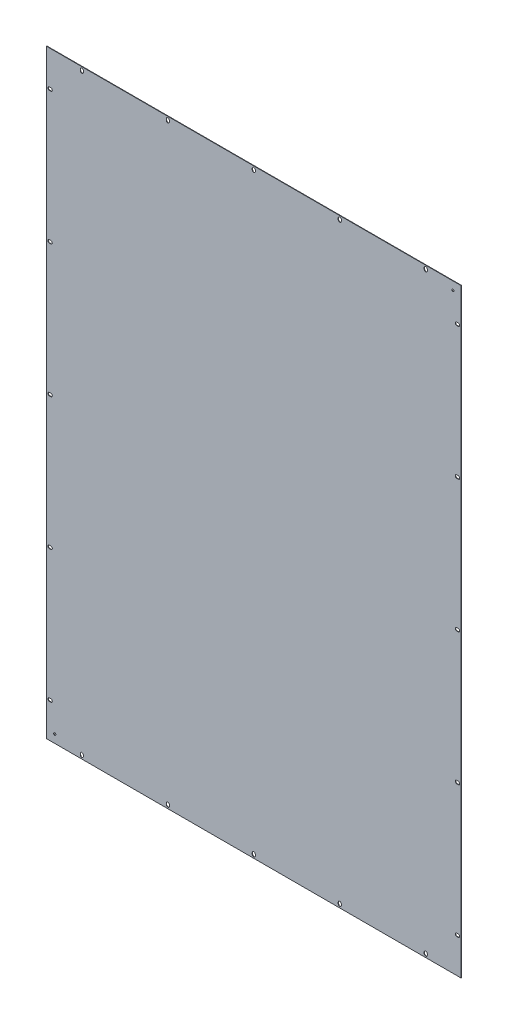
from build123d import *

# Parameters (mm, degrees)
SKETCH_1_W          = 940
SKETCH_1_H          = 1360
EXTRUDE_1_DEPTH     = 1
SKETCH_3_R          = 2.5
CUT_EXTRUDE_2_DEPTH = 10
CUT_EXTRUDE_3_DEPTH = 10


with BuildPart() as part:
    # 草图1 → 凸台-拉伸1 (new body)
    with BuildSketch(Plane.XY):
        Rectangle(SKETCH_1_W, SKETCH_1_H)
    extrude(amount=EXTRUDE_1_DEPTH)

    # 草图3 → 切除-拉伸2 (cut)
    with BuildSketch(Plane(origin=(0, 0, 0), x_dir=(-1, 0, 0), z_dir=(0, 0, -1))):
        with Locations((451.5, -661.5)):
            Circle(SKETCH_3_R)
        with Locations((-451.5, 661.5)):
            Circle(SKETCH_3_R)
    extrude(amount=-CUT_EXTRUDE_2_DEPTH, mode=Mode.SUBTRACT)

    # 草图4 → 切除-拉伸3 (cut)
    with BuildSketch(Plane(origin=(0, 0, 0), x_dir=(-1, 0, 0), z_dir=(0, 0, -1))):
        with BuildLine():
            Line((3.5, -670.5), (3.5, -673.5))
            ThreePointArc((3.5, -673.5), (0, -677), (-3.5, -673.5))
            Line((-3.5, -673.5), (-3.5, -670.5))
            ThreePointArc((-3.5, -670.5), (0, -667), (3.5, -670.5))
        make_face()
        with BuildLine():
            Line((-191.5, -670.5), (-191.5, -673.5))
            ThreePointArc((-191.5, -673.5), (-195, -677), (-198.5, -673.5))
            Line((-198.5, -673.5), (-198.5, -670.5))
            ThreePointArc((-198.5, -670.5), (-195, -667), (-191.5, -670.5))
        make_face()
        with BuildLine():
            Line((-386.5, -670.5), (-386.5, -673.5))
            ThreePointArc((-386.5, -673.5), (-390, -677), (-393.5, -673.5))
            Line((-393.5, -673.5), (-393.5, -670.5))
            ThreePointArc((-393.5, -670.5), (-390, -667), (-386.5, -670.5))
        make_face()
        with BuildLine():
            Line((386.5, -670.5), (386.5, -673.5))
            ThreePointArc((386.5, -673.5), (390, -677), (393.5, -673.5))
            Line((393.5, -673.5), (393.5, -670.5))
            ThreePointArc((393.5, -670.5), (390, -667), (386.5, -670.5))
        make_face()
        with BuildLine():
            Line((191.5, -670.5), (191.5, -673.5))
            ThreePointArc((191.5, -673.5), (195, -677), (198.5, -673.5))
            Line((198.5, -673.5), (198.5, -670.5))
            ThreePointArc((198.5, -670.5), (195, -667), (191.5, -670.5))
        make_face()
        with BuildLine():
            Line((-460.5, -3.5), (-463.5, -3.5))
            ThreePointArc((-463.5, -3.5), (-467, 0), (-463.5, 3.5))
            Line((-463.5, 3.5), (-460.5, 3.5))
            ThreePointArc((-460.5, 3.5), (-457, 0), (-460.5, -3.5))
        make_face()
        with BuildLine():
            Line((-460.5, 296.5), (-463.5, 296.5))
            ThreePointArc((-463.5, 296.5), (-467, 300), (-463.5, 303.5))
            Line((-463.5, 303.5), (-460.5, 303.5))
            ThreePointArc((-460.5, 303.5), (-457, 300), (-460.5, 296.5))
        make_face()
        with BuildLine():
            Line((-460.5, 596.5), (-463.5, 596.5))
            ThreePointArc((-463.5, 596.5), (-467, 600), (-463.5, 603.5))
            Line((-463.5, 603.5), (-460.5, 603.5))
            ThreePointArc((-460.5, 603.5), (-457, 600), (-460.5, 596.5))
        make_face()
        with BuildLine():
            Line((-460.5, -596.5), (-463.5, -596.5))
            ThreePointArc((-463.5, -596.5), (-467, -600), (-463.5, -603.5))
            Line((-463.5, -603.5), (-460.5, -603.5))
            ThreePointArc((-460.5, -603.5), (-457, -600), (-460.5, -596.5))
        make_face()
        with BuildLine():
            Line((-460.5, -296.5), (-463.5, -296.5))
            ThreePointArc((-463.5, -296.5), (-467, -300), (-463.5, -303.5))
            Line((-463.5, -303.5), (-460.5, -303.5))
            ThreePointArc((-460.5, -303.5), (-457, -300), (-460.5, -296.5))
        make_face()
        with BuildLine():
            Line((191.5, 670.5), (191.5, 673.5))
            ThreePointArc((191.5, 673.5), (195, 677), (198.5, 673.5))
            Line((198.5, 673.5), (198.5, 670.5))
            ThreePointArc((198.5, 670.5), (195, 667), (191.5, 670.5))
        make_face()
        with BuildLine():
            Line((386.5, 670.5), (386.5, 673.5))
            ThreePointArc((386.5, 673.5), (390, 677), (393.5, 673.5))
            Line((393.5, 673.5), (393.5, 670.5))
            ThreePointArc((393.5, 670.5), (390, 667), (386.5, 670.5))
        make_face()
        with BuildLine():
            Line((-386.5, 670.5), (-386.5, 673.5))
            ThreePointArc((-386.5, 673.5), (-390, 677), (-393.5, 673.5))
            Line((-393.5, 673.5), (-393.5, 670.5))
            ThreePointArc((-393.5, 670.5), (-390, 667), (-386.5, 670.5))
        make_face()
        with BuildLine():
            Line((-191.5, 670.5), (-191.5, 673.5))
            ThreePointArc((-191.5, 673.5), (-195, 677), (-198.5, 673.5))
            Line((-198.5, 673.5), (-198.5, 670.5))
            ThreePointArc((-198.5, 670.5), (-195, 667), (-191.5, 670.5))
        make_face()
        with BuildLine():
            Line((3.5, 670.5), (3.5, 673.5))
            ThreePointArc((3.5, 673.5), (0, 677), (-3.5, 673.5))
            Line((-3.5, 673.5), (-3.5, 670.5))
            ThreePointArc((-3.5, 670.5), (0, 667), (3.5, 670.5))
        make_face()
        with BuildLine():
            Line((460.5, 596.5), (463.5, 596.5))
            ThreePointArc((463.5, 596.5), (467, 600), (463.5, 603.5))
            Line((463.5, 603.5), (460.5, 603.5))
            ThreePointArc((460.5, 603.5), (457, 600), (460.5, 596.5))
        make_face()
        with BuildLine():
            Line((460.5, -296.5), (463.5, -296.5))
            ThreePointArc((463.5, -296.5), (467, -300), (463.5, -303.5))
            Line((463.5, -303.5), (460.5, -303.5))
            ThreePointArc((460.5, -303.5), (457, -300), (460.5, -296.5))
        make_face()
        with BuildLine():
            Line((460.5, -596.5), (463.5, -596.5))
            ThreePointArc((463.5, -596.5), (467, -600), (463.5, -603.5))
            Line((463.5, -603.5), (460.5, -603.5))
            ThreePointArc((460.5, -603.5), (457, -600), (460.5, -596.5))
        make_face()
        with BuildLine():
            Line((460.5, 296.5), (463.5, 296.5))
            ThreePointArc((463.5, 296.5), (467, 300), (463.5, 303.5))
            Line((463.5, 303.5), (460.5, 303.5))
            ThreePointArc((460.5, 303.5), (457, 300), (460.5, 296.5))
        make_face()
        with BuildLine():
            Line((460.5, -3.5), (463.5, -3.5))
            ThreePointArc((463.5, -3.5), (467, 0), (463.5, 3.5))
            Line((463.5, 3.5), (460.5, 3.5))
            ThreePointArc((460.5, 3.5), (457, 0), (460.5, -3.5))
        make_face()
    extrude(amount=-CUT_EXTRUDE_3_DEPTH, mode=Mode.SUBTRACT)


solid = part.part
